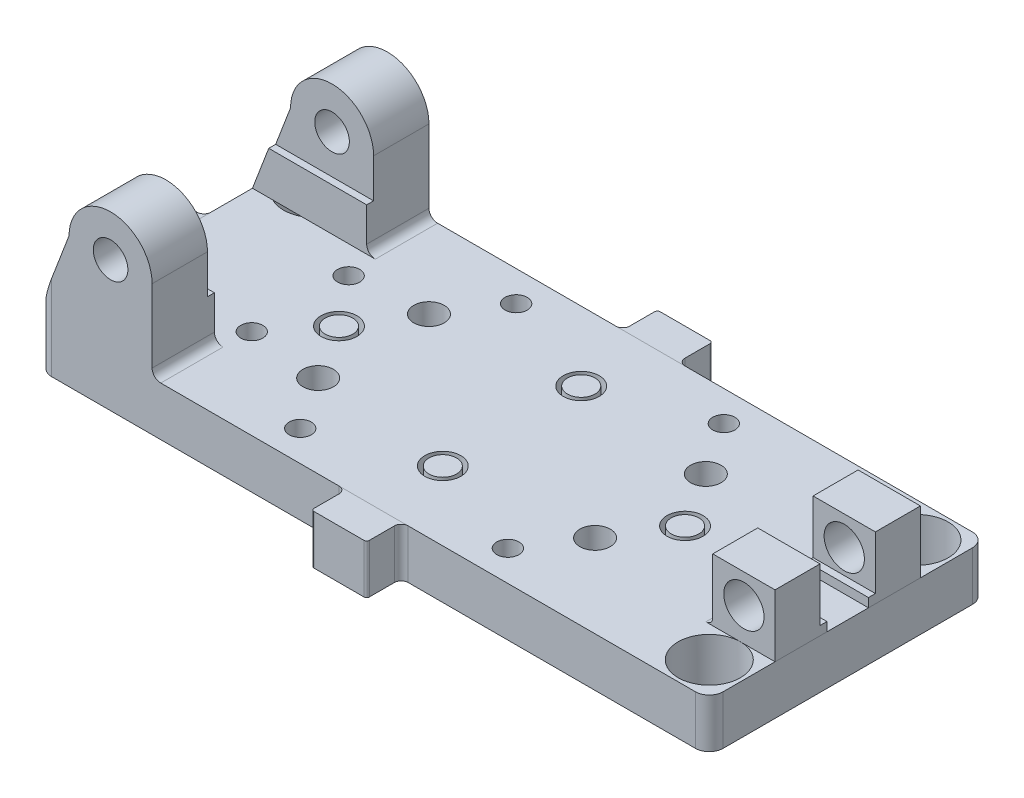
from build123d import *

# Parameters (mm, degrees)
SKETCH1_R                  = 12.5
BOSS_EXTRUDE1_DEPTH        = 100
CUT_EXTRUDE1_DEPTH         = 284.18962695
CUT_EXTRUDE1_DEPTH_BACK    = 284.18962695
SKETCH3_R                  = 14.553943417
BOSS_EXTRUDE2_DEPTH        = 52.5
CUT_EXTRUDE3_DEPTH         = 284.18962695
CUT_EXTRUDE3_DEPTH_BACK    = 284.18962695
CUT_EXTRUDE4_DEPTH         = 284.18962695
CUT_EXTRUDE4_DEPTH_BACK    = 284.18962695
SKETCH5_R                  = 8
SKETCH5_R_2                = 13
SKETCH5_R_3                = 10
SKETCH5_R_4                = 11
SKETCH5_W                  = 20.521758455
SKETCH5_H                  = 25
BOSS_EXTRUDE5_DEPTH        = 17.720286
BOSS_EXTRUDE5_DEPTH_BACK   = 17.720286
BOSS_EXTRUDE5_2_DEPTH      = 17.720286
BOSS_EXTRUDE5_2_DEPTH_BACK = 17.720286
BOSS_EXTRUDE5_3_DEPTH      = 17.720286
BOSS_EXTRUDE5_3_DEPTH_BACK = 17.720286
CUT_EXTRUDE5_DEPTH         = 17.720286
CUT_EXTRUDE5_DEPTH_BACK    = 314.960916539
SKETCH7_R                  = 22.5
FILLET11_R                 = 10


with BuildPart() as part:
    # Sketch1 → Boss-Extrude1 (new, symmetric)
    # profile 1 of 2: a face of its own
    with BuildSketch(Plane.XY):
        with BuildLine():
            Line((-231.799247234, 17.720286162), (-231.799247234, -17.720286162))
            Line((-231.799247234, -17.720286162), (242.501846041, -17.720286162))
            Line((242.501846041, -17.720286162), (242.501846041, 17.720286162))
            Line((242.501846041, 17.720286162), (-153.753855421, 17.720286162))
            ThreePointArc((-153.753855421, 17.720286162), (-158.170546609, 19.549739553), (-160, 23.966430741))
            Line((-160, 23.966430741), (-160, 76.720286162))
            ThreePointArc((-160, 76.720286162), (-190, 106.720286162), (-220, 76.720286162))
            ThreePointArc((-220, 76.720286162), (-218.824763602, 68.405660295), (-215.391133112, 60.742477825))
            Line((-215.391133112, 60.742477825), (-231.799247234, 17.720286162))
        make_face()
        with Locations((-190, 76.720286162)):
            Circle(SKETCH1_R, mode=Mode.SUBTRACT)
    # profile 2 of 2: a face of its own
    with BuildSketch(Plane.XY):
        with BuildLine():
            Line((-242.501846041, -17.279713838), (-242.501846041, -17.720286162))
            Line((-242.501846041, -17.720286162), (-231.799247234, -17.720286162))
            Line((-231.799247234, -17.720286162), (-231.799247234, 17.720286162))
            Line((-231.799247234, 17.720286162), (-215.391133112, 60.742477825))
            ThreePointArc((-215.391133112, 60.742477825), (-218.824763602, 68.405660295), (-220, 76.720286162))
            Line((-220, 76.720286162), (-242.501846041, 17.720286162))
            Line((-242.501846041, 17.720286162), (-242.501846041, -17.279713838))
        make_face()
    extrude(amount=BOSS_EXTRUDE1_DEPTH, both=True)

    # Sketch2 → Cut-Extrude1 (cut, two sides: drawn at the far end of the back side and taken through both)
    with BuildSketch(Plane(origin=(0, 0, 0), x_dir=(0, 0, -1), z_dir=(1, 0, 0)).offset(-CUT_EXTRUDE1_DEPTH_BACK)):
        Polygon((-60, 106.720286162), (-60, 48.584551896), (-55, 48.584551896), (-55, 17.720286162), (55, 17.720286162), (55, 48.584551896), (60, 48.584551896), (60, 106.720286162), align=None)
    extrude(amount=CUT_EXTRUDE1_DEPTH + CUT_EXTRUDE1_DEPTH_BACK, mode=Mode.SUBTRACT)

    # Sketch5 → Cut-Extrude4 (cut, two sides: drawn at the far end of the back side and taken through both)
    # profile 1 of 15: a face of its own
    with BuildSketch(Plane(origin=(0, 0, 0), x_dir=(1, 0, 0), z_dir=(0, 1, 0)).offset(-CUT_EXTRUDE4_DEPTH_BACK)):
        with Locations(Location((-153, 35, 0), (0, 0, 270))):
            Circle(SKETCH5_R)
    # profile 2 of 15: a face of its own
    with BuildSketch(Plane(origin=(0, 0, 0), x_dir=(1, 0, 0), z_dir=(0, 1, 0)).offset(-CUT_EXTRUDE4_DEPTH_BACK)):
        with Locations(Location((-153, -35, 0), (0, 0, 270))):
            Circle(SKETCH5_R)
    # profile 3 of 15: a face of its own
    with BuildSketch(Plane(origin=(0, 0, 0), x_dir=(1, 0, 0), z_dir=(0, 1, 0)).offset(-CUT_EXTRUDE4_DEPTH_BACK)):
        with Locations(Location((-125, 0, 0), (0, 0, 270))):
            Circle(SKETCH5_R_2)
        with Locations(Location((-125, 0, 0), (0, 0, 270))):
            Circle(SKETCH5_R_3, mode=Mode.SUBTRACT)
    # profile 4 of 15: a face of its own
    with BuildSketch(Plane(origin=(0, 0, 0), x_dir=(1, 0, 0), z_dir=(0, 1, 0)).offset(-CUT_EXTRUDE4_DEPTH_BACK)):
        with Locations(Location((-100, 40, 0), (0, 0, 270))):
            Circle(SKETCH5_R_4)
    # profile 5 of 15: a face of its own
    with BuildSketch(Plane(origin=(0, 0, 0), x_dir=(1, 0, 0), z_dir=(0, 1, 0)).offset(-CUT_EXTRUDE4_DEPTH_BACK)):
        with Locations(Location((-100, -40, 0), (0, 0, 270))):
            Circle(SKETCH5_R_4)
    # profile 6 of 15: a face of its own
    with BuildSketch(Plane(origin=(0, 0, 0), x_dir=(1, 0, 0), z_dir=(0, 1, 0)).offset(-CUT_EXTRUDE4_DEPTH_BACK)):
        with Locations(Location((0, 50, 0), (0, 0, 270))):
            Circle(SKETCH5_R_2)
        with Locations(Location((0, 50, 0), (0, 0, 270))):
            Circle(SKETCH5_R_3, mode=Mode.SUBTRACT)
    # profile 7 of 15: a face of its own
    with BuildSketch(Plane(origin=(0, 0, 0), x_dir=(1, 0, 0), z_dir=(0, 1, 0)).offset(-CUT_EXTRUDE4_DEPTH_BACK)):
        with Locations(Location((0, -50, 0), (0, 0, 270))):
            Circle(SKETCH5_R_2)
        with Locations(Location((0, -50, 0), (0, 0, 270))):
            Circle(SKETCH5_R_3, mode=Mode.SUBTRACT)
    # profile 8 of 15: a face of its own
    with BuildSketch(Plane(origin=(0, 0, 0), x_dir=(1, 0, 0), z_dir=(0, 1, 0)).offset(-CUT_EXTRUDE4_DEPTH_BACK)):
        with Locations(Location((75, -78, 0), (0, 0, 180))):
            Circle(SKETCH5_R)
    # profile 9 of 15: a face of its own
    with BuildSketch(Plane(origin=(0, 0, 0), x_dir=(1, 0, 0), z_dir=(0, 1, 0)).offset(-CUT_EXTRUDE4_DEPTH_BACK)):
        with Locations(Location((100, -40, 0), (0, 0, 180))):
            Circle(SKETCH5_R_4)
    # profile 10 of 15: a face of its own
    with BuildSketch(Plane(origin=(0, 0, 0), x_dir=(1, 0, 0), z_dir=(0, 1, 0)).offset(-CUT_EXTRUDE4_DEPTH_BACK)):
        with Locations(Location((-75, 78, 0), (0, 0, 270))):
            Circle(SKETCH5_R)
    # profile 11 of 15: a face of its own
    with BuildSketch(Plane(origin=(0, 0, 0), x_dir=(1, 0, 0), z_dir=(0, 1, 0)).offset(-CUT_EXTRUDE4_DEPTH_BACK)):
        with Locations(Location((-75, -78, 0), (0, 0, 270))):
            Circle(SKETCH5_R)
    # profile 12 of 15: a face of its own
    with BuildSketch(Plane(origin=(0, 0, 0), x_dir=(1, 0, 0), z_dir=(0, 1, 0)).offset(-CUT_EXTRUDE4_DEPTH_BACK)):
        with Locations(Location((125, 0, 0), (0, 0, 180))):
            Circle(SKETCH5_R_2)
        with Locations(Location((125, 0, 0), (0, 0, 180))):
            Circle(SKETCH5_R_3, mode=Mode.SUBTRACT)
    # profile 13 of 15: a face of its own
    with BuildSketch(Plane(origin=(0, 0, 0), x_dir=(1, 0, 0), z_dir=(0, 1, 0)).offset(-CUT_EXTRUDE4_DEPTH_BACK)):
        with Locations(Location((100, 40, 0), (0, 0, 180))):
            Circle(SKETCH5_R_4)
    # profile 14 of 15: a face of its own
    with BuildSketch(Plane(origin=(0, 0, 0), x_dir=(1, 0, 0), z_dir=(0, 1, 0)).offset(-CUT_EXTRUDE4_DEPTH_BACK)):
        with Locations(Location((75, 78, 0), (0, 0, 180))):
            Circle(SKETCH5_R)
    # profile 15 of 15: a face of its own
    with BuildSketch(Plane(origin=(0, 0, 0), x_dir=(1, 0, 0), z_dir=(0, 1, 0)).offset(-CUT_EXTRUDE4_DEPTH_BACK)):
        with Locations((-10.260879228, 112.5)):
            Rectangle(SKETCH5_W, SKETCH5_H)
    extrude(amount=CUT_EXTRUDE4_DEPTH + CUT_EXTRUDE4_DEPTH_BACK, mode=Mode.SUBTRACT)


with BuildPart() as body_2:
    # Sketch3 → Boss-Extrude2 (new, symmetric)
    with BuildSketch(Plane.XY):
        with BuildLine():
            Line((242.501846041, 17.720286162), (192.501846041, 17.720286162))
            ThreePointArc((192.501846041, 17.720286162), (196.037379947, 19.184752256), (197.501846041, 22.720286162))
            Line((197.501846041, 22.720286162), (197.501846041, 62.720286162))
            Line((197.501846041, 62.720286162), (242.501846041, 62.720286162))
            Line((242.501846041, 62.720286162), (242.501846041, 17.720286162))
        make_face()
        with Locations((220.001846041, 41.720286162)):
            Circle(SKETCH3_R, mode=Mode.SUBTRACT)
    extrude(amount=BOSS_EXTRUDE2_DEPTH, both=True)

    # Sketch4 → Cut-Extrude3 (cut, two sides: drawn at the far end of the back side and taken through both)
    with BuildSketch(Plane(origin=(0, 0, 0), x_dir=(0, 0, -1), z_dir=(1, 0, 0)).offset(-CUT_EXTRUDE3_DEPTH_BACK)):
        Polygon((-20, 62.720286162), (-20, 24.157412536), (-15, 24.157412536), (-15, 17.720286162), (15, 17.720286162), (15, 24.157412536), (20, 24.157412536), (20, 62.720286162), align=None)
    extrude(amount=CUT_EXTRUDE3_DEPTH + CUT_EXTRUDE3_DEPTH_BACK, mode=Mode.SUBTRACT)


with BuildPart() as cut_extrude3_piece_1:
    # of the separate pieces the step leaves, piece 1, a body of its own (cut_extrude3_pieces)
    add(body_2.part.solids().sort_by_distance((242.501846041, 17.720286162, 15))[0])


with BuildPart() as cut_extrude3_piece_2:
    # of the separate pieces the step leaves, piece 2, a body of its own (cut_extrude3_pieces)
    add(body_2.part.solids().sort_by_distance((242.501846041, 17.720286162, -52.5))[0])


with BuildPart() as cut_extrude4_piece_1:
    # of the separate pieces the step leaves, piece 1, a body of its own (cut_extrude4_pieces)
    add(part.part.solids().sort_by_distance((-220, 76.720286162, 100))[0])

    # Sketch7 → Cut-Extrude5 (cut, two sides: drawn at the far end of the back side and taken through both)
    with BuildSketch(Plane(origin=(0, 0, 0), x_dir=(1, 0, 0), z_dir=(0, 1, 0)).offset(-CUT_EXTRUDE5_DEPTH_BACK)):
        with Locations(Location((217.501846041, -75, 0), (0, 0, 270))):
            Circle(SKETCH7_R)
        with Locations(Location((217.501846041, 75, 0), (0, 0, 180))):
            Circle(SKETCH7_R)
        with Locations(Location((-217.501846041, 75, 0), (0, 0, 270))):
            Circle(SKETCH7_R)
        with Locations(Location((-217.501846041, -75, 0), (0, 0, 117.266044451))):
            Circle(SKETCH7_R)
    extrude(amount=CUT_EXTRUDE5_DEPTH + CUT_EXTRUDE5_DEPTH_BACK, mode=Mode.SUBTRACT)

    # Fillet11
    fillet11_edges = [cut_extrude4_piece_1.edges().sort_by_distance(p)[0] for p in [
        (-242.501846041, 0, 100),
        (242.501846041, 0, -100),
        (242.501846041, 0, 100),
        (-242.501846041, 0, -100),
    ]]
    fillet(fillet11_edges, radius=FILLET11_R)


with BuildPart() as cut_extrude4_piece_2:
    # of the separate pieces the step leaves, piece 2, a body of its own (cut_extrude4_pieces)
    add(part.part.solids().sort_by_distance((0, 17.720286162, -40))[0])


with BuildPart() as cut_extrude4_piece_3:
    # of the separate pieces the step leaves, piece 3, a body of its own (cut_extrude4_pieces)
    add(part.part.solids().sort_by_distance((0, 17.720286162, 60))[0])


with BuildPart() as cut_extrude4_piece_4:
    # of the separate pieces the step leaves, piece 4, a body of its own (cut_extrude4_pieces)
    add(part.part.solids().sort_by_distance((-125, 17.720286162, 10))[0])


with BuildPart() as cut_extrude4_piece_5:
    # of the separate pieces the step leaves, piece 5, a body of its own (cut_extrude4_pieces)
    add(part.part.solids().sort_by_distance((115, 17.720286162, 0))[0])


with BuildPart() as body_8:
    # Sketch6 → Boss-Extrude5 (new, two sides: drawn at the far end of the back side and taken through both)
    with BuildSketch(Plane(origin=(0, 0, 0), x_dir=(1, 0, 0), z_dir=(0, 1, 0)).offset(-BOSS_EXTRUDE5_DEPTH_BACK)):
        with BuildLine():
            Line((-247.501846041, 20), (-265.501846041, 20))
            ThreePointArc((-265.501846041, 20), (-266.916059604, 19.414213562), (-267.501846041, 18))
            Line((-267.501846041, 18), (-267.501846041, -18))
            ThreePointArc((-267.501846041, -18), (-266.916059604, -19.414213562), (-265.501846041, -20))
            Line((-265.501846041, -20), (-247.501846041, -20))
            ThreePointArc((-247.501846041, -20), (-243.966312135, -21.464466094), (-242.501846041, -25))
            Line((-242.501846041, -25), (-242.501846041, 25))
            ThreePointArc((-242.501846041, 25), (-243.966312135, 21.464466094), (-247.501846041, 20))
        make_face()
    extrude(amount=BOSS_EXTRUDE5_DEPTH + BOSS_EXTRUDE5_DEPTH_BACK)


with BuildPart() as body_9:
    # Sketch6 → Boss-Extrude5 2 (new, two sides: drawn at the far end of the back side and taken through both)
    with BuildSketch(Plane(origin=(0, 0, 0), x_dir=(1, 0, 0), z_dir=(0, 1, 0)).offset(-BOSS_EXTRUDE5_2_DEPTH_BACK)):
        with BuildLine():
            Line((25, 100), (-25, 100))
            ThreePointArc((-25, 100), (-21.464466094, 101.464466094), (-20, 105))
            Line((-20, 105), (-20, 123))
            ThreePointArc((-20, 123), (-19.414213562, 124.414213562), (-18, 125))
            Line((-18, 125), (18, 125))
            ThreePointArc((18, 125), (19.414213562, 124.414213562), (20, 123))
            Line((20, 123), (20, 105))
            ThreePointArc((20, 105), (21.464466094, 101.464466094), (25, 100))
        make_face()
    extrude(amount=BOSS_EXTRUDE5_2_DEPTH + BOSS_EXTRUDE5_2_DEPTH_BACK)


with BuildPart() as body_10:
    # Sketch6 → Boss-Extrude5 3 (new, two sides: drawn at the far end of the back side and taken through both)
    with BuildSketch(Plane(origin=(0, 0, 0), x_dir=(1, 0, 0), z_dir=(0, 1, 0)).offset(-BOSS_EXTRUDE5_3_DEPTH_BACK)):
        with BuildLine():
            Line((20, -105), (20, -123))
            ThreePointArc((20, -123), (19.414213562, -124.414213562), (18, -125))
            Line((18, -125), (-18, -125))
            ThreePointArc((-18, -125), (-19.414213562, -124.414213562), (-20, -123))
            Line((-20, -123), (-20, -105))
            ThreePointArc((-20, -105), (-21.464466094, -101.464466094), (-25, -100))
            Line((-25, -100), (25, -100))
            ThreePointArc((25, -100), (21.464466094, -101.464466094), (20, -105))
        make_face()
    extrude(amount=BOSS_EXTRUDE5_3_DEPTH + BOSS_EXTRUDE5_3_DEPTH_BACK)


solid = Compound([cut_extrude3_piece_1.part, cut_extrude3_piece_2.part, cut_extrude4_piece_1.part, cut_extrude4_piece_2.part, cut_extrude4_piece_3.part, cut_extrude4_piece_4.part, cut_extrude4_piece_5.part, body_8.part, body_9.part, body_10.part])
